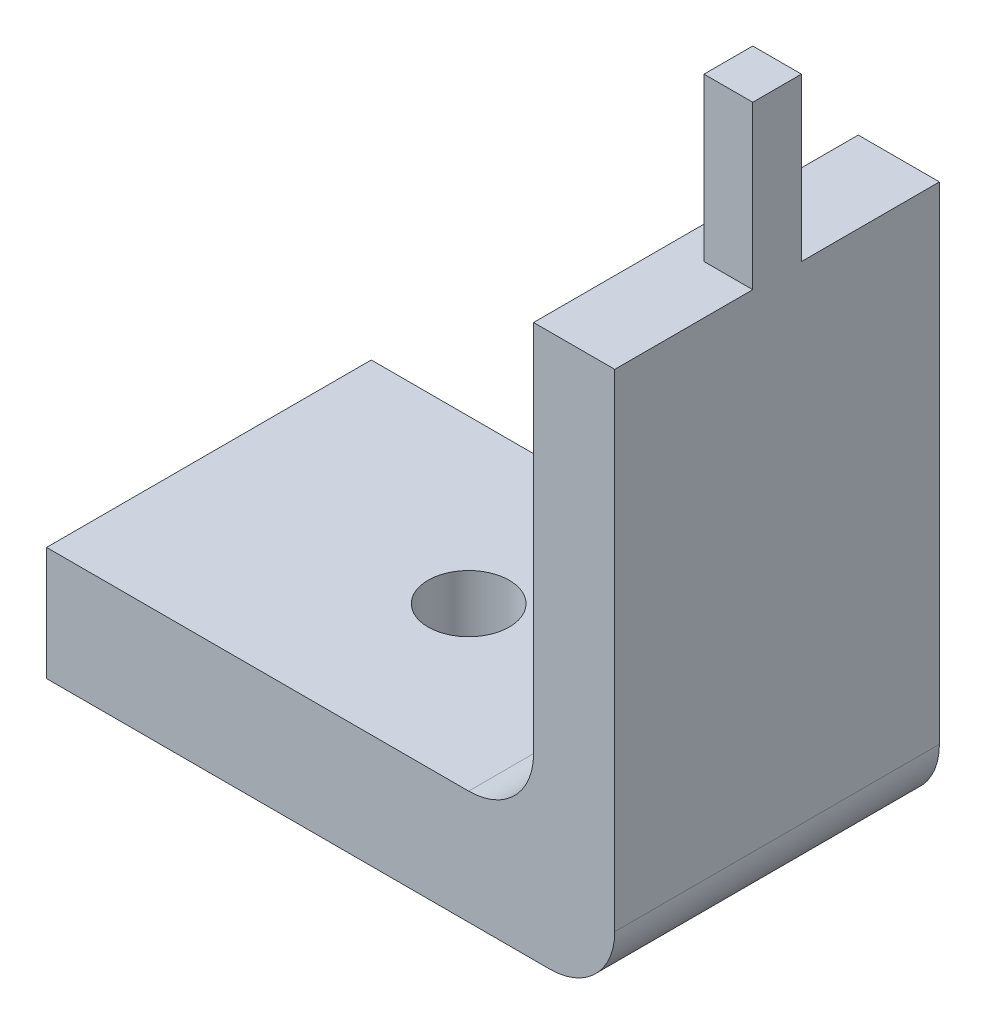
from build123d import *

# Parameters (mm, degrees)
BOSS_EXTRUDE1_DEPTH   = 10
SKETCH2_W             = 1.5
SKETCH2_H             = 5
BOSS_EXTRUDE2_DEPTH   = 1.5
FILLET1_R             = 2
M3_TAPPED_HOLE1_D     = 2.5
M3_TAPPED_HOLE1_DEPTH = 8.5
M3_TAPPED_HOLE1_TIP   = 0.751075774


with BuildPart() as part:
    # Sketch1 → Boss-Extrude1 (new body)
    with BuildSketch(Plane.XY):
        Polygon((0, 0), (17.5, 0), (17.5, 17), (15, 17), (15, 3.5), (0, 3.5), align=None)
    extrude(amount=BOSS_EXTRUDE1_DEPTH)

    # Sketch2 → Boss-Extrude2 (add)
    with BuildSketch(Plane(origin=(17.5, 0, 0), x_dir=(0, 0, -1), z_dir=(1, 0, 0))):
        with Locations((-5, 19.5)):
            Rectangle(SKETCH2_W, SKETCH2_H)
    extrude(amount=-BOSS_EXTRUDE2_DEPTH)

    # Fillet1
    fillet1_edges = [part.edges().sort_by_distance(p)[0] for p in [
        (15, 3.5, 5),
        (17.5, 0, 5),
    ]]
    fillet(fillet1_edges, radius=FILLET1_R)

    # M3 Tapped Hole1
    with Locations(Plane(origin=(0, 3.5, 0), x_dir=(1, 0, 0), z_dir=(0, 1, 0))):
        with Locations((8, -5)):
            Hole(M3_TAPPED_HOLE1_D / 2, depth=M3_TAPPED_HOLE1_DEPTH)
            with Locations((0, 0, -(M3_TAPPED_HOLE1_DEPTH + M3_TAPPED_HOLE1_TIP / 2))):  # 118° drill point
                Cone(0, M3_TAPPED_HOLE1_D / 2, M3_TAPPED_HOLE1_TIP, mode=Mode.SUBTRACT)


solid = part.part
